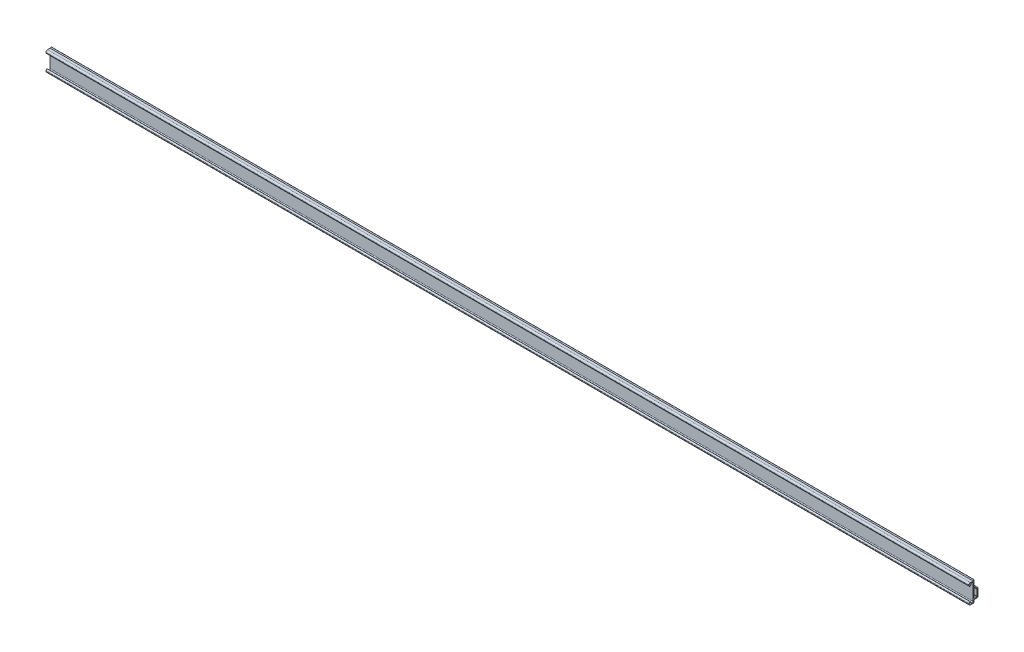
from build123d import *

# Parameters (mm, degrees)
BOSS_EXTRUDE1_DEPTH = 915


with BuildPart() as part:
    # Sketch1 → Boss-Extrude1 (new body)
    with BuildSketch(Plane(origin=(-422.5, 0, 0), x_dir=(0, -1, 0), z_dir=(-1, 0, 0))):
        with BuildLine():
            Line((-755.11, 454.95), (-755.11, 452.15))
            ThreePointArc((-755.11, 452.15), (-755.183223305, 451.973223305), (-755.36, 451.9))
            Line((-755.36, 451.9), (-762.01, 451.9))
            Line((-762.01, 451.9), (-762.01, 452.7))
            Line((-762.01, 452.7), (-762.56, 452.7))
            ThreePointArc((-762.56, 452.7), (-762.736776695, 452.626776695), (-762.81, 452.45))
            Line((-762.81, 452.45), (-762.81, 451.35))
            ThreePointArc((-762.81, 451.35), (-762.736776695, 451.173223305), (-762.56, 451.1))
            Line((-762.56, 451.1), (-755.31, 451.1))
            ThreePointArc((-755.31, 451.1), (-754.602893219, 451.392893219), (-754.31, 452.1))
            Line((-754.31, 452.1), (-754.31, 453.373491886))
            ThreePointArc((-754.31, 453.373491886), (-753.775028159, 454.665028159), (-752.483491886, 455.2))
            Line((-752.483491886, 455.2), (-752.41, 455.2))
            ThreePointArc((-752.41, 455.2), (-751.702893219, 455.492893219), (-751.41, 456.2))
            Line((-751.41, 456.2), (-751.41, 458.6))
            ThreePointArc((-751.41, 458.6), (-751.849339828, 459.660660172), (-752.91, 460.1))
            Line((-752.91, 460.1), (-753.31, 460.1))
            ThreePointArc((-753.31, 460.1), (-754.301183271, 459.232498012), (-753.572659626, 458.135111446))
            Line((-753.572659626, 458.135111446), (-752.947340374, 457.964888554))
            ThreePointArc((-752.947340374, 457.964888554), (-752.218816729, 456.867501988), (-753.21, 456))
            Line((-753.21, 456), (-768.909810447, 456))
            ThreePointArc((-768.909810447, 456), (-769.900988627, 456.867463908), (-769.172544211, 457.964868369))
            Line((-769.172544211, 457.964868369), (-768.547266236, 458.135131631))
            ThreePointArc((-768.547266236, 458.135131631), (-767.81882182, 459.232536092), (-768.81, 460.1))
            Line((-768.81, 460.1), (-769.21, 460.1))
            ThreePointArc((-769.21, 460.1), (-770.270660172, 459.660660172), (-770.71, 458.6))
            Line((-770.71, 458.6), (-770.71, 456))
            ThreePointArc((-770.71, 456), (-770.959658895, 455.534896264), (-771.353431907, 455.183337075))
            ThreePointArc((-771.353431907, 455.183337075), (-771.39533621, 455.130932577), (-771.394682745, 455.06383731))
            ThreePointArc((-771.394682745, 455.06383731), (-771.317838721, 454.956126495), (-771.196783129, 454.902720811))
            ThreePointArc((-771.196783129, 454.902720811), (-771.165207963, 454.903064362), (-771.135314114, 454.913236231))
            ThreePointArc((-771.135314114, 454.913236231), (-770.541156786, 455.135665686), (-769.91, 455.2))
            Line((-769.91, 455.2), (-755.36, 455.2))
            ThreePointArc((-755.36, 455.2), (-755.183223305, 455.126776695), (-755.11, 454.95))
        make_face()
    extrude(amount=-BOSS_EXTRUDE1_DEPTH)


solid = part.part
